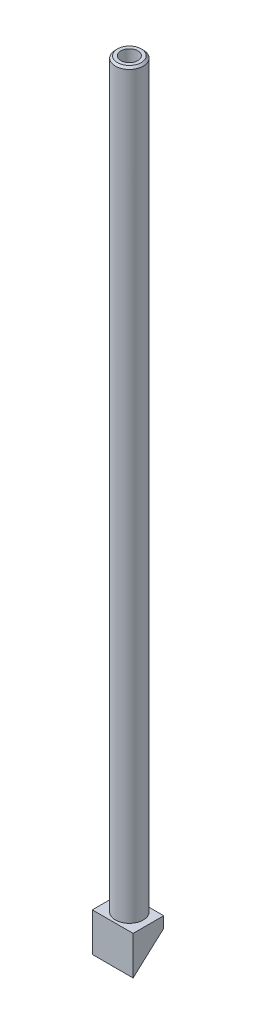
from build123d import *

# Parameters (mm, degrees)
SKETCH1_R                = 205
SKETCH1_R_2              = 125
BOSS_EXTRUDE1_DEPTH      = 10900
BOSS_EXTRUDE2_START      = 2
SKETCH2_R                = 205
BOSS_EXTRUDE2_DEPTH      = 2
CHAMFER1_SIZE            = 30
BOSS_EXTRUDE3_DEPTH      = 300
BOSS_EXTRUDE3_DEPTH_BACK = 300


with BuildPart() as part:
    # Sketch1 → Boss-Extrude1 (new body)
    with BuildSketch(Plane(origin=(0, 0, 0), x_dir=(1, 0, 0), z_dir=(0, 1, 0))):
        with Locations(Location((0, 0, 0), (0, 0, 90))):
            Circle(SKETCH1_R)
        with Locations(Location((0, 0, 0), (0, 0, 90))):
            Circle(SKETCH1_R_2, mode=Mode.SUBTRACT)
    extrude(amount=BOSS_EXTRUDE1_DEPTH)

    # Sketch2 → Boss-Extrude2 (add)
    with BuildSketch(Plane.XZ.offset(BOSS_EXTRUDE2_START)):
        with Locations(Location((0, 0, 0), (0, 0, 270))):
            Circle(SKETCH2_R)
    extrude(amount=-BOSS_EXTRUDE2_DEPTH)

    # Chamfer1
    chamfer1_edges = [part.edges().sort_by_distance(p)[0] for p in [
        (0, 10900, 205),
    ]]
    chamfer(chamfer1_edges, length=CHAMFER1_SIZE)

    # Sketch3 → Boss-Extrude3 (add, two sides: drawn at the far end of the back side and taken through both)
    with BuildSketch(Plane(origin=(0, 0, 0), x_dir=(0, 0, -1), z_dir=(1, 0, 0)).offset(-BOSS_EXTRUDE3_DEPTH_BACK)):
        Polygon((205, -2), (205, -163.463903414), (-245, -569.910586712), (-245, -2), align=None)
    extrude(amount=BOSS_EXTRUDE3_DEPTH + BOSS_EXTRUDE3_DEPTH_BACK)


solid = part.part
